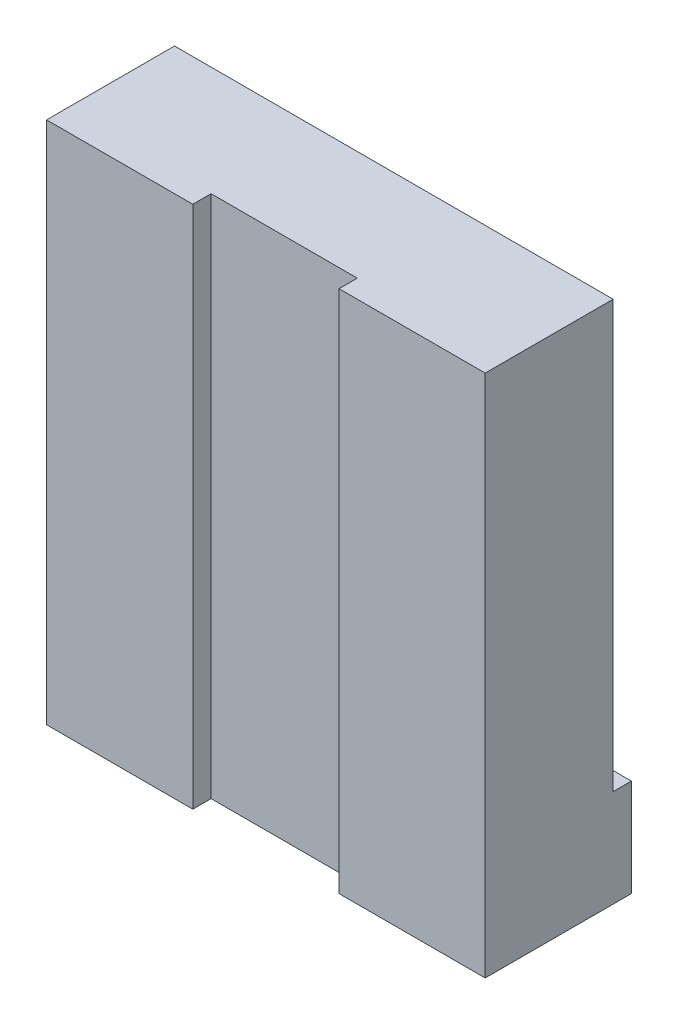
from build123d import *

# Parameters (mm, degrees)
SKETCH_1_W          = 36
SKETCH_1_H          = 43
EXTRUDE_1_DEPTH     = 6
SKETCH_2_W          = 12
SKETCH_2_H          = 43
CUT_EXTRUDE_1_DEPTH = 1.5
SKETCH_3_W          = 30.5
SKETCH_3_H          = 43
CUT_EXTRUDE_2_DEPTH = 1.5
SKETCH_4_W          = 36
SKETCH_4_H          = 35
CUT_EXTRUDE_3_DEPTH = 1.5


with BuildPart() as part:
    # 草图1 → 凸台-拉伸1 (new, symmetric)
    with BuildSketch(Plane.XY):
        Rectangle(SKETCH_1_W, SKETCH_1_H)
    extrude(amount=EXTRUDE_1_DEPTH, both=True)

    # 草图2 → 切除-拉伸1 (cut)
    with BuildSketch(Plane.XY.offset(6)):
        Rectangle(SKETCH_2_W, SKETCH_2_H)
    extrude(amount=-CUT_EXTRUDE_1_DEPTH, mode=Mode.SUBTRACT)

    # 草图3 → 切除-拉伸2 (cut)
    with BuildSketch(Plane(origin=(0, 0, -6), x_dir=(-1, 0, 0), z_dir=(0, 0, -1))):
        Rectangle(SKETCH_3_W, SKETCH_3_H)
    extrude(amount=-CUT_EXTRUDE_2_DEPTH, mode=Mode.SUBTRACT)

    # 草图4 → 切除-拉伸3 (cut)
    with BuildSketch(Plane(origin=(0, 0, -6), x_dir=(-1, 0, 0), z_dir=(0, 0, -1))):
        with Locations((0, 4)):
            Rectangle(SKETCH_4_W, SKETCH_4_H)
    extrude(amount=-CUT_EXTRUDE_3_DEPTH, mode=Mode.SUBTRACT)


solid = part.part
